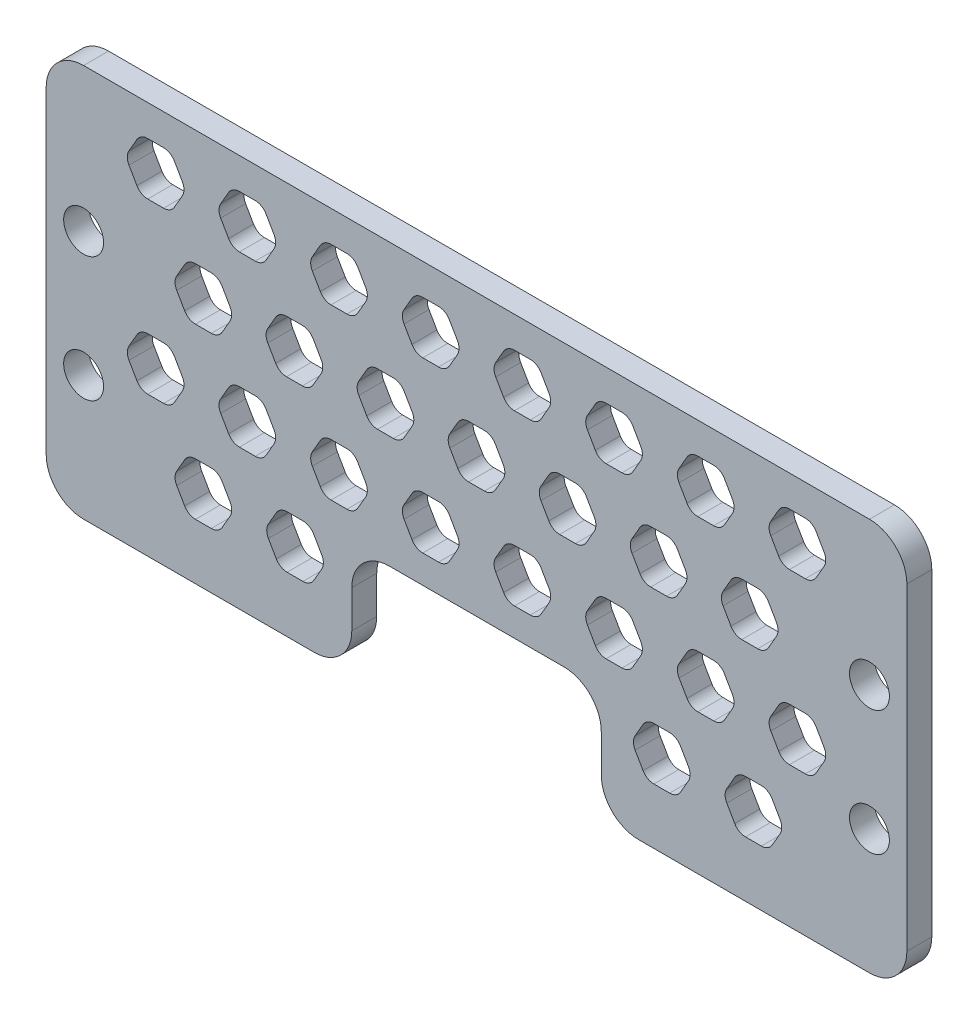
SolidWorks part; units mm, degrees
material "Thornel Mat VMA"
ref_plane "前视基准面" through (0, 0, 0) normal (0, 0, 1) x (1, 0, 0)
ref_plane "上视基准面" through (0, 0, 0) normal (0, 1, 0) x (1, 0, 0)
ref_plane "右视基准面" through (0, 0, 0) normal (1, 0, 0) x (0, 0, -1)
sketch "草图1" plane through (0, 0, 0) normal (0, 0, 1) x (1, 0, 0)
  line L0 (0, 15.75) -> (0, -6.75) construction
  line L1 (-34.5, 15.75) -> (34.5, 15.75)
  line L2 (-34.5, 15.75) -> (-34.5, -15.75)
  line L3 (-34.5, -15.75) -> (-10, -15.75)
  line L4 (34.5, 15.75) -> (34.5, -15.75)
  line L5 (-34.5, 15.75) -> (34.5, -15.75) construction
  line L6 (-34.5, -15.75) -> (34.5, 15.75) construction
  line L7 (-31.5, 4.25) -> (-31.5, -5.75) construction
  line L8 (31.5, 4.25) -> (31.5, -5.75) construction
  line L9 (-10, -15.75) -> (-10, -6.75)
  line L10 (10, -15.75) -> (10, -6.75)
  line L11 (-10, -6.75) -> (10, -6.75)
  line L12 (10, -15.75) -> (34.5, -15.75)
  circle A0 centre (-31.5, 4.25) radius 1.6
  circle A1 centre (-31.5, -5.75) radius 1.6
  circle A2 centre (31.5, -5.75) radius 1.6
  circle A3 centre (31.5, 4.25) radius 1.6
  point P0 (0, 0)
  dimension "D1" = 69
  dimension "D3" = 3.2
  dimension "D2" = 31.5
  dimension "D4" = 10
  dimension "D5" = 3
  dimension "D6" = 20
  dimension "D7" = 9
  dimension "D8" = 11.5
extrude "凸台-拉伸1" add sketch "草图1" along normal blind 2
sketch "草图2" plane through (0, 0, 2) normal (0, 0, 1) x (1, 0, 0)
  line L0 (-28.149, 11.15) -> (-26.9365, 13.25)
  line L1 (-26.9365, 13.25) -> (-24.5117, 13.25)
  line L2 (-24.5117, 13.25) -> (-23.2992, 11.15)
  line L3 (-23.2992, 11.15) -> (-24.5117, 9.05)
  line L4 (-24.5117, 9.05) -> (-26.9365, 9.05)
  line L5 (-26.9365, 9.05) -> (-28.149, 11.15)
  line L6 (-19.5868, 9.05) -> (-20.7992, 11.15)
  line L7 (-20.7992, 11.15) -> (-19.5868, 13.25)
  line L8 (-19.5868, 13.25) -> (-17.1619, 13.25)
  line L9 (-17.1619, 13.25) -> (-15.9495, 11.15)
  line L10 (-15.9495, 11.15) -> (-17.1619, 9.05)
  line L11 (-17.1619, 9.05) -> (-19.5868, 9.05)
  line L12 (-12.237, 9.05) -> (-13.4495, 11.15)
  line L13 (-13.4495, 11.15) -> (-12.237, 13.25)
  line L14 (-12.237, 13.25) -> (-9.8122, 13.25)
  line L15 (-9.8122, 13.25) -> (-8.5997, 11.15)
  line L16 (-8.5997, 11.15) -> (-9.8122, 9.05)
  line L17 (-9.8122, 9.05) -> (-12.237, 9.05)
  line L18 (-4.8873, 9.05) -> (-6.0997, 11.15)
  line L19 (-6.0997, 11.15) -> (-4.8873, 13.25)
  line L20 (-4.8873, 13.25) -> (-2.4624, 13.25)
  line L21 (-2.4624, 13.25) -> (-1.25, 11.15)
  line L22 (-1.25, 11.15) -> (-2.4624, 9.05)
  line L23 (-2.4624, 9.05) -> (-4.8873, 9.05)
  line L24 (2.4624, 9.05) -> (1.25, 11.15)
  line L25 (1.25, 11.15) -> (2.4624, 13.25)
  line L26 (2.4624, 13.25) -> (4.8873, 13.25)
  line L27 (4.8873, 13.25) -> (6.0997, 11.15)
  line L28 (6.0997, 11.15) -> (4.8873, 9.05)
  line L29 (4.8873, 9.05) -> (2.4624, 9.05)
  line L30 (9.8122, 9.05) -> (8.5997, 11.15)
  line L31 (8.5997, 11.15) -> (9.8122, 13.25)
  line L32 (9.8122, 13.25) -> (12.237, 13.25)
  line L33 (12.237, 13.25) -> (13.4495, 11.15)
  line L34 (13.4495, 11.15) -> (12.237, 9.05)
  line L35 (12.237, 9.05) -> (9.8122, 9.05)
  line L36 (17.1619, 9.05) -> (15.9495, 11.15)
  line L37 (15.9495, 11.15) -> (17.1619, 13.25)
  line L38 (17.1619, 13.25) -> (19.5868, 13.25)
  line L39 (19.5868, 13.25) -> (20.7992, 11.15)
  line L40 (20.7992, 11.15) -> (19.5868, 9.05)
  line L41 (19.5868, 9.05) -> (17.1619, 9.05)
  line L42 (24.5117, 9.05) -> (23.2992, 11.15)
  line L43 (23.2992, 11.15) -> (24.5117, 13.25)
  line L44 (24.5117, 13.25) -> (26.9365, 13.25)
  line L45 (26.9365, 13.25) -> (28.149, 11.15)
  line L46 (28.149, 11.15) -> (26.9365, 9.05)
  line L47 (26.9365, 9.05) -> (24.5117, 9.05)
  line L48 (0, 15.75) -> (0, -6.75) construction
  line L49 (34.5, 15.75) -> (-34.5, 15.75) construction
  line L50 (-10, -6.75) -> (10, -6.75) construction
  line L51 (-24.3241, 4.3749) -> (-23.1117, 6.4749)
  line L52 (-23.1117, 6.4749) -> (-20.6868, 6.4749)
  line L53 (-20.6868, 6.4749) -> (-19.4744, 4.3749)
  line L54 (-19.4744, 4.3749) -> (-20.6868, 2.2749)
  line L55 (-20.6868, 2.2749) -> (-23.1117, 2.2749)
  line L56 (-23.1117, 2.2749) -> (-24.3241, 4.3749)
  line L57 (-15.8119, 2.2749) -> (-17.0244, 4.3749)
  line L58 (-17.0244, 4.3749) -> (-15.8119, 6.4749)
  line L59 (-15.8119, 6.4749) -> (-13.387, 6.4749)
  line L60 (-13.387, 6.4749) -> (-12.1746, 4.3749)
  line L61 (-12.1746, 4.3749) -> (-13.387, 2.2749)
  line L62 (-13.387, 2.2749) -> (-15.8119, 2.2749)
  line L63 (-8.5122, 2.2749) -> (-9.7246, 4.3749)
  line L64 (-9.7246, 4.3749) -> (-8.5122, 6.4749)
  line L65 (-8.5122, 6.4749) -> (-6.0873, 6.4749)
  line L66 (-6.0873, 6.4749) -> (-4.8749, 4.3749)
  line L67 (-4.8749, 4.3749) -> (-6.0873, 2.2749)
  line L68 (-6.0873, 2.2749) -> (-8.5122, 2.2749)
  line L69 (-1.2124, 2.2749) -> (-2.4249, 4.3749)
  line L70 (-2.4249, 4.3749) -> (-1.2124, 6.4749)
  line L71 (-1.2124, 6.4749) -> (1.2124, 6.4749)
  line L72 (1.2124, 6.4749) -> (2.4249, 4.3749)
  line L73 (2.4249, 4.3749) -> (1.2124, 2.2749)
  line L74 (1.2124, 2.2749) -> (-1.2124, 2.2749)
  line L75 (6.0873, 2.2749) -> (4.8749, 4.3749)
  line L76 (4.8749, 4.3749) -> (6.0873, 6.4749)
  line L77 (6.0873, 6.4749) -> (8.5122, 6.4749)
  line L78 (8.5122, 6.4749) -> (9.7246, 4.3749)
  line L79 (9.7246, 4.3749) -> (8.5122, 2.2749)
  line L80 (8.5122, 2.2749) -> (6.0873, 2.2749)
  line L81 (13.387, 2.2749) -> (12.1746, 4.3749)
  line L82 (12.1746, 4.3749) -> (13.387, 6.4749)
  line L83 (13.387, 6.4749) -> (15.8119, 6.4749)
  line L84 (15.8119, 6.4749) -> (17.0244, 4.3749)
  line L85 (17.0244, 4.3749) -> (15.8119, 2.2749)
  line L86 (15.8119, 2.2749) -> (13.387, 2.2749)
  line L87 (20.6868, 2.2749) -> (19.4744, 4.3749)
  line L88 (19.4744, 4.3749) -> (20.6868, 6.4749)
  line L89 (20.6868, 6.4749) -> (23.1117, 6.4749)
  line L90 (23.1117, 6.4749) -> (24.3241, 4.3749)
  line L91 (24.3241, 4.3749) -> (23.1117, 2.2749)
  line L92 (23.1117, 2.2749) -> (20.6868, 2.2749)
  line L93 (-24.3241, 4.3749) -> (-19.4744, 4.3749) construction
  line L94 (-26.9365, -4.5003) -> (-28.149, -2.4003)
  line L95 (-28.149, -2.4003) -> (-26.9365, -0.3003)
  line L96 (-26.9365, -0.3003) -> (-24.5117, -0.3003)
  line L97 (-24.5117, -0.3003) -> (-23.2992, -2.4003)
  line L98 (-23.2992, -2.4003) -> (-24.5117, -4.5003)
  line L99 (-24.5117, -4.5003) -> (-26.9365, -4.5003)
  line L100 (-19.5868, -4.5003) -> (-20.7992, -2.4003)
  line L101 (-20.7992, -2.4003) -> (-19.5868, -0.3003)
  line L102 (-19.5868, -0.3003) -> (-17.1619, -0.3003)
  line L103 (-17.1619, -0.3003) -> (-15.9495, -2.4003)
  line L104 (-15.9495, -2.4003) -> (-17.1619, -4.5003)
  line L105 (-17.1619, -4.5003) -> (-19.5868, -4.5003)
  line L106 (-12.237, -4.5003) -> (-13.4495, -2.4003)
  line L107 (-13.4495, -2.4003) -> (-12.237, -0.3003)
  line L108 (-12.237, -0.3003) -> (-9.8122, -0.3003)
  line L109 (-9.8122, -0.3003) -> (-8.5997, -2.4003)
  line L110 (-8.5997, -2.4003) -> (-9.8122, -4.5003)
  line L111 (-9.8122, -4.5003) -> (-12.237, -4.5003)
  line L112 (-4.8873, -4.5003) -> (-6.0997, -2.4003)
  line L113 (-6.0997, -2.4003) -> (-4.8873, -0.3003)
  line L114 (-4.8873, -0.3003) -> (-2.4624, -0.3003)
  line L115 (-2.4624, -0.3003) -> (-1.25, -2.4003)
  line L116 (-1.25, -2.4003) -> (-2.4624, -4.5003)
  line L117 (-2.4624, -4.5003) -> (-4.8873, -4.5003)
  line L118 (2.4624, -4.5003) -> (1.25, -2.4003)
  line L119 (1.25, -2.4003) -> (2.4624, -0.3003)
  line L120 (2.4624, -0.3003) -> (4.8873, -0.3003)
  line L121 (4.8873, -0.3003) -> (6.0997, -2.4003)
  line L122 (6.0997, -2.4003) -> (4.8873, -4.5003)
  line L123 (4.8873, -4.5003) -> (2.4624, -4.5003)
  line L124 (9.8122, -4.5003) -> (8.5997, -2.4003)
  line L125 (8.5997, -2.4003) -> (9.8122, -0.3003)
  line L126 (9.8122, -0.3003) -> (12.237, -0.3003)
  line L127 (12.237, -0.3003) -> (13.4495, -2.4003)
  line L128 (13.4495, -2.4003) -> (12.237, -4.5003)
  line L129 (12.237, -4.5003) -> (9.8122, -4.5003)
  line L130 (17.1619, -4.5003) -> (15.9495, -2.4003)
  line L131 (15.9495, -2.4003) -> (17.1619, -0.3003)
  line L132 (17.1619, -0.3003) -> (19.5868, -0.3003)
  line L133 (19.5868, -0.3003) -> (20.7992, -2.4003)
  line L134 (20.7992, -2.4003) -> (19.5868, -4.5003)
  line L135 (19.5868, -4.5003) -> (17.1619, -4.5003)
  line L136 (24.5117, -4.5003) -> (23.2992, -2.4003)
  line L137 (23.2992, -2.4003) -> (24.5117, -0.3003)
  line L138 (24.5117, -0.3003) -> (26.9365, -0.3003)
  line L139 (26.9365, -0.3003) -> (28.149, -2.4003)
  line L140 (28.149, -2.4003) -> (26.9365, -4.5003)
  line L141 (26.9365, -4.5003) -> (24.5117, -4.5003)
  line L142 (-24.3241, -9.1754) -> (-23.1117, -7.0754)
  line L143 (-23.1117, -7.0754) -> (-20.6868, -7.0754)
  line L144 (-20.6868, -7.0754) -> (-19.4744, -9.1754)
  line L145 (-19.4744, -9.1754) -> (-20.6868, -11.2754)
  line L146 (-20.6868, -11.2754) -> (-23.1117, -11.2754)
  line L147 (-23.1117, -11.2754) -> (-24.3241, -9.1754)
  line L166 (-15.7619, -11.2754) -> (-16.9744, -9.1754)
  line L167 (-16.9744, -9.1754) -> (-15.7619, -7.0754)
  line L168 (-15.7619, -7.0754) -> (-13.337, -7.0754)
  line L169 (-13.337, -7.0754) -> (-12.1246, -9.1754)
  line L170 (-12.1246, -9.1754) -> (-13.337, -11.2754)
  line L171 (-13.337, -11.2754) -> (-15.7619, -11.2754)
  line L172 (-8.4122, -11.2754) -> (-9.6246, -9.1754) construction
  line L173 (-9.6246, -9.1754) -> (-8.4122, -7.0754) construction
  line L174 (-8.4122, -7.0754) -> (-5.9873, -7.0754) construction
  line L175 (-5.9873, -7.0754) -> (-4.7749, -9.1754) construction
  line L176 (-4.7749, -9.1754) -> (-5.9873, -11.2754) construction
  line L177 (-5.9873, -11.2754) -> (-8.4122, -11.2754) construction
  line L178 (-1.0624, -11.2754) -> (-2.2749, -9.1754) construction
  line L179 (-2.2749, -9.1754) -> (-1.0624, -7.0754) construction
  line L180 (-1.0624, -7.0754) -> (1.3624, -7.0754) construction
  line L181 (1.3624, -7.0754) -> (2.5749, -9.1754) construction
  line L182 (2.5749, -9.1754) -> (1.3624, -11.2754) construction
  line L183 (1.3624, -11.2754) -> (-1.0624, -11.2754) construction
  line L184 (6.2873, -11.2754) -> (5.0749, -9.1754) construction
  line L185 (5.0749, -9.1754) -> (6.2873, -7.0754) construction
  line L186 (6.2873, -7.0754) -> (8.7122, -7.0754) construction
  line L187 (8.7122, -7.0754) -> (9.9246, -9.1754) construction
  line L188 (9.9246, -9.1754) -> (8.7122, -11.2754) construction
  line L189 (8.7122, -11.2754) -> (6.2873, -11.2754) construction
  line L190 (13.637, -11.2754) -> (12.4246, -9.1754)
  line L191 (12.4246, -9.1754) -> (13.637, -7.0754)
  line L192 (13.637, -7.0754) -> (16.0619, -7.0754)
  line L193 (16.0619, -7.0754) -> (17.2744, -9.1754)
  line L194 (17.2744, -9.1754) -> (16.0619, -11.2754)
  line L195 (16.0619, -11.2754) -> (13.637, -11.2754)
  line L196 (20.9868, -11.2754) -> (19.7744, -9.1754)
  line L197 (19.7744, -9.1754) -> (20.9868, -7.0754)
  line L198 (20.9868, -7.0754) -> (23.4117, -7.0754)
  line L199 (23.4117, -7.0754) -> (24.6241, -9.1754)
  line L200 (24.6241, -9.1754) -> (23.4117, -11.2754)
  line L201 (23.4117, -11.2754) -> (20.9868, -11.2754)
  circle A0 centre (-25.7241, 11.15) radius 2.4249 construction
  circle A1 centre (-21.8992, 4.3749) radius 2.4249 construction
  circle A2 centre (-21.8992, -9.1754) radius 2.4249 construction
  point P158 (0, 0)
  dimension "D1" = 4.2
  dimension "D5" = 1.4
  dimension "D10" = 2.5
  dimension "D3" = 2.5
  dimension "D4" = 2.5
  dimension "D6" = 2.5
  dimension "D8" = 2
  dimension "D9" = 2.5
  dimension "D11" = 7
  dimension "D12" = 2.5
  dimension "D2" = 8
  dimension "D7" = 7
extrude "切除-拉伸1" cut sketch "草图2" against normal through all
fillet "R1 镂空圆角" radius 1 119 edges at (-28.149, 11.15, 1) (-26.9365, 13.25, 1) (-24.5117, 13.25, 1) (-24.5117, 9.05, 1) (-15.7619, -7.0754, 1) (-13.337, -7.0754, 1) (-12.1246, -9.1754, 1) (-15.7619, -11.2754, 1) (-16.9744, -9.1754, 1) (-24.3241, -9.1754, 1) (-19.4744, -9.1754, 1) (-20.6868, -11.2754, 1) (-23.1117, -11.2754, 1) (26.9365, -0.3003, 1) (28.149, -2.4003, 1) (26.9365, -4.5003, 1) (24.5117, -4.5003, 1) (17.1619, -0.3003, 1) (19.5868, -0.3003, 1) (20.7992, -2.4003, 1) (17.1619, -4.5003, 1) (15.9495, -2.4003, 1) (9.8122, -0.3003, 1) (12.237, -4.5003, 1) (9.8122, -4.5003, 1) (8.5997, -2.4003, 1) (2.4624, -0.3003, 1) (4.8873, -0.3003, 1) (4.8873, -4.5003, 1) (2.4624, -4.5003, 1) (1.25, -2.4003, 1) (-4.8873, -0.3003, 1) (-2.4624, -0.3003, 1) (-2.4624, -4.5003, 1) (-4.8873, -4.5003, 1) (-6.0997, -2.4003, 1) (-9.8122, -0.3003, 1) (-8.5997, -2.4003, 1) (-9.8122, -4.5003, 1) (-13.4495, -2.4003, 1) (13.637, -7.0754, 1) (16.0619, -7.0754, 1) (17.2744, -9.1754, 1) (13.637, -11.2754, 1) (12.4246, -9.1754, 1) (20.9868, -7.0754, 1) (23.4117, -7.0754, 1) (24.6241, -9.1754, 1) (23.4117, -11.2754, 1) (19.7744, -9.1754, 1) (13.4495, 11.15, 1) (12.237, 9.05, 1) (17.1619, 13.25, 1) (19.5868, 13.25, 1) (19.5868, 9.05, 1) (17.1619, 9.05, 1) (15.9495, 11.15, 1) (24.5117, 13.25, 1) (26.9365, 13.25, 1) (28.149, 11.15, 1) (26.9365, 9.05, 1) (24.5117, 9.05, 1) (-20.6868, 6.4749, 1) (-20.6868, 2.2749, 1) (-23.1117, 2.2749, 1) (2.4624, 13.25, 1) (4.8873, 13.25, 1) (6.0997, 11.15, 1) (4.8873, 9.05, 1) (2.4624, 9.05, 1) (-2.4624, 13.25, 1) (-1.25, 11.15, 1) (-2.4624, 9.05, 1) (-4.8873, 9.05, 1) (-12.237, 13.25, 1) (-9.8122, 13.25, 1) (-8.5997, 11.15, 1) (-9.8122, 9.05, 1) (-12.237, 9.05, 1) (-17.1619, 13.25, 1) (-15.9495, 11.15, 1) (-17.1619, 9.05, 1) (-19.5868, 9.05, 1) (-20.7992, 11.15, 1) (6.0873, 6.4749, 1) (8.5122, 2.2749, 1) (4.8749, 4.3749, 1) (15.8119, 6.4749, 1) (17.0244, 4.3749, 1) (15.8119, 2.2749, 1) (13.387, 2.2749, 1) (20.6868, 6.4749, 1) (24.3241, 4.3749, 1) (23.1117, 2.2749, 1) (19.4744, 4.3749, 1) (-19.5868, -0.3003, 1) (-17.1619, -0.3003, 1) (-17.1619, -4.5003, 1) (-19.5868, -4.5003, 1) (-20.7992, -2.4003, 1) (-1.2124, 6.4749, 1) (1.2124, 6.4749, 1) (-1.2124, 2.2749, 1) (-2.4249, 4.3749, 1) (-8.5122, 6.4749, 1) (-4.8749, 4.3749, 1) (-6.0873, 2.2749, 1) (-8.5122, 2.2749, 1) (-9.7246, 4.3749, 1) (-15.8119, 6.4749, 1) (-12.1746, 4.3749, 1) (-13.387, 2.2749, 1) (-15.8119, 2.2749, 1) (-17.0244, 4.3749, 1) (-26.9365, -0.3003, 1) (-24.5117, -0.3003, 1) (-24.5117, -4.5003, 1) (-26.9365, -4.5003, 1) (-23.2992, 11.15, 1)
fillet "R3 外缘圆角" radius 3 8 edges at (10, -15.75, 1) (10, -6.75, 1) (-10, -6.75, 1) (-34.5, -15.75, 1) (-34.5, 15.75, 1) (34.5, 15.75, 1) (34.5, -15.75, 1) (-10, -15.75, 1)
